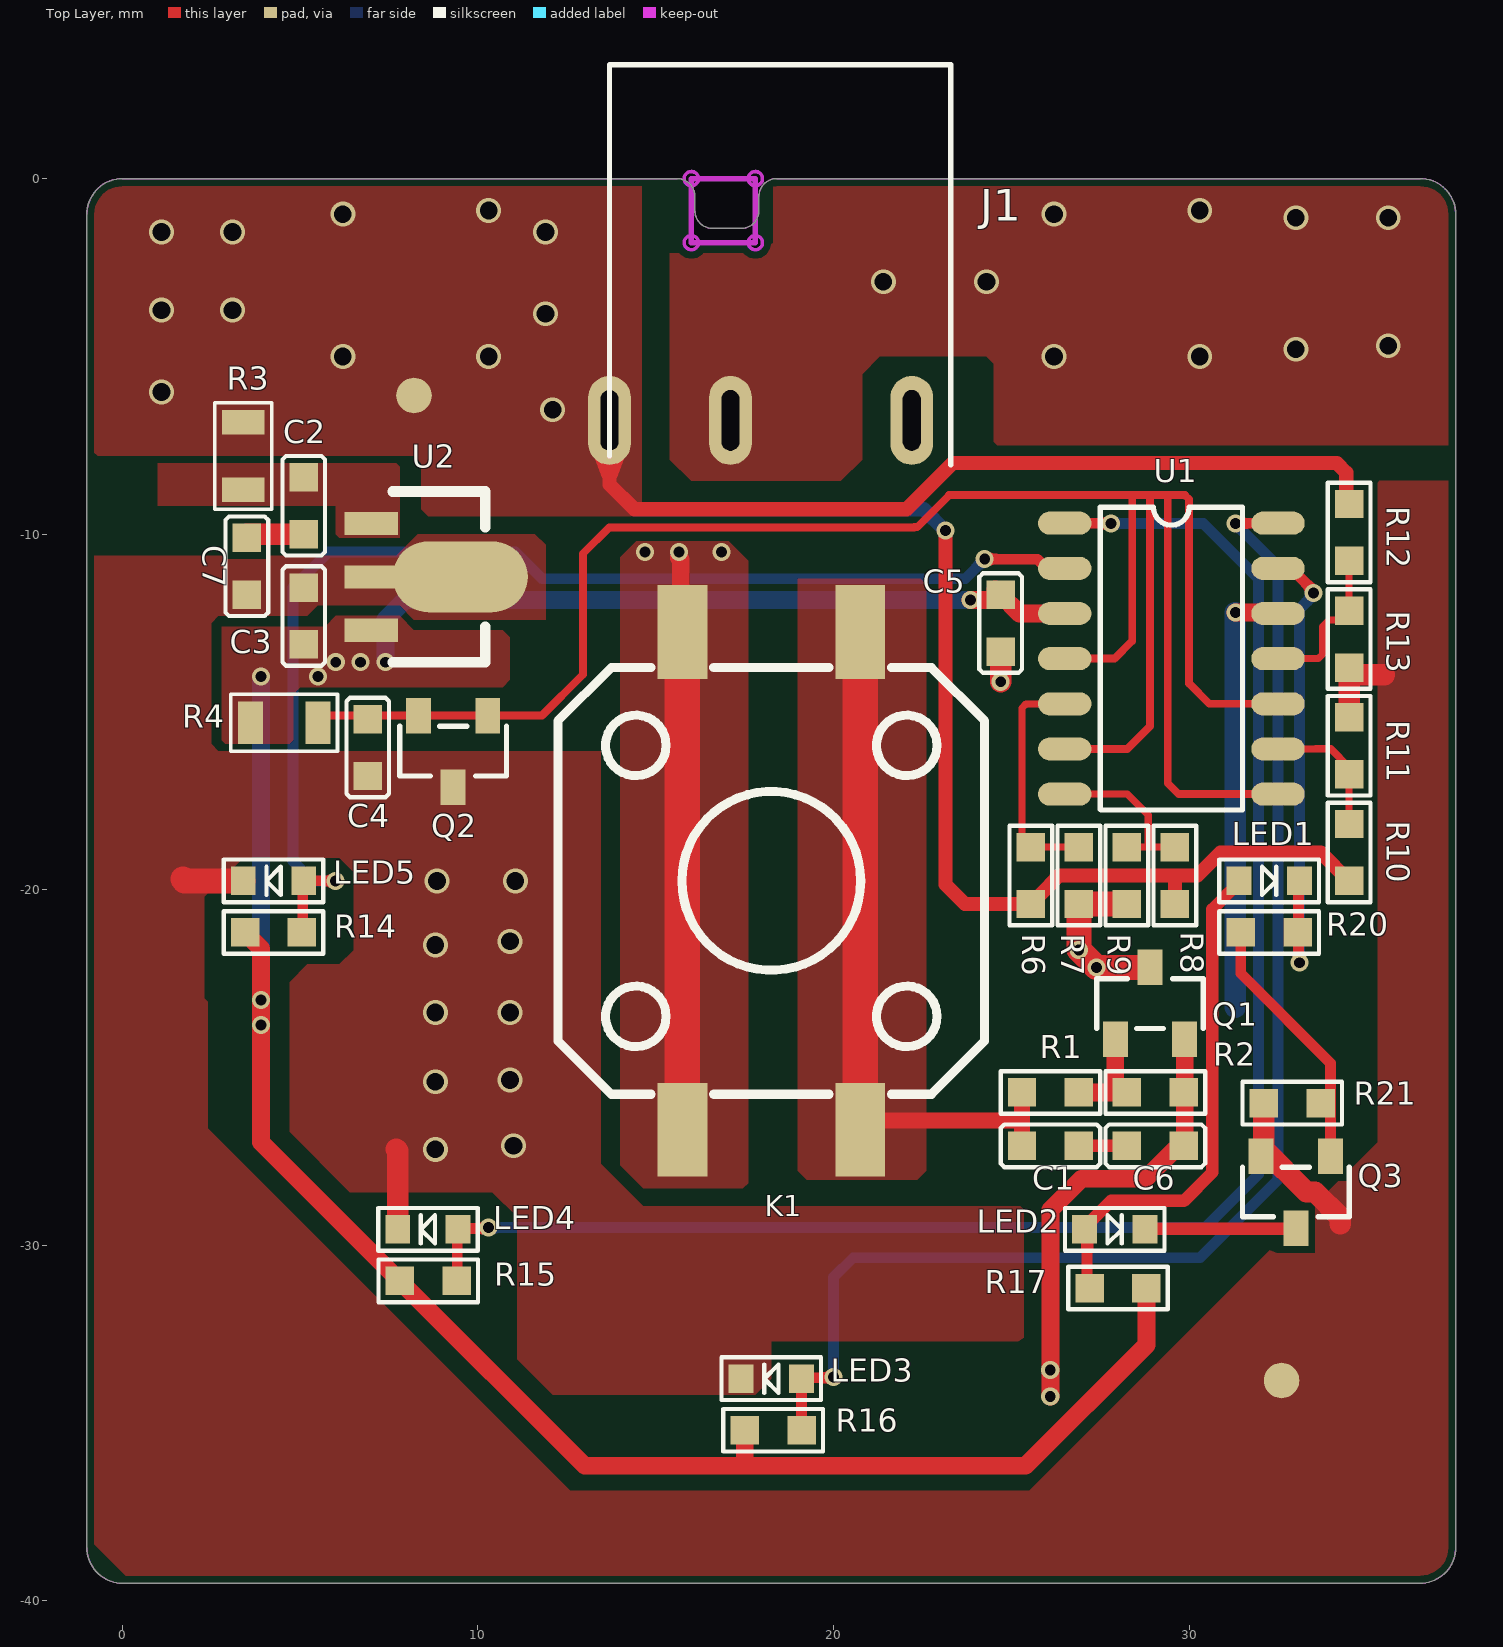
[diagram p0: Top Layer view]
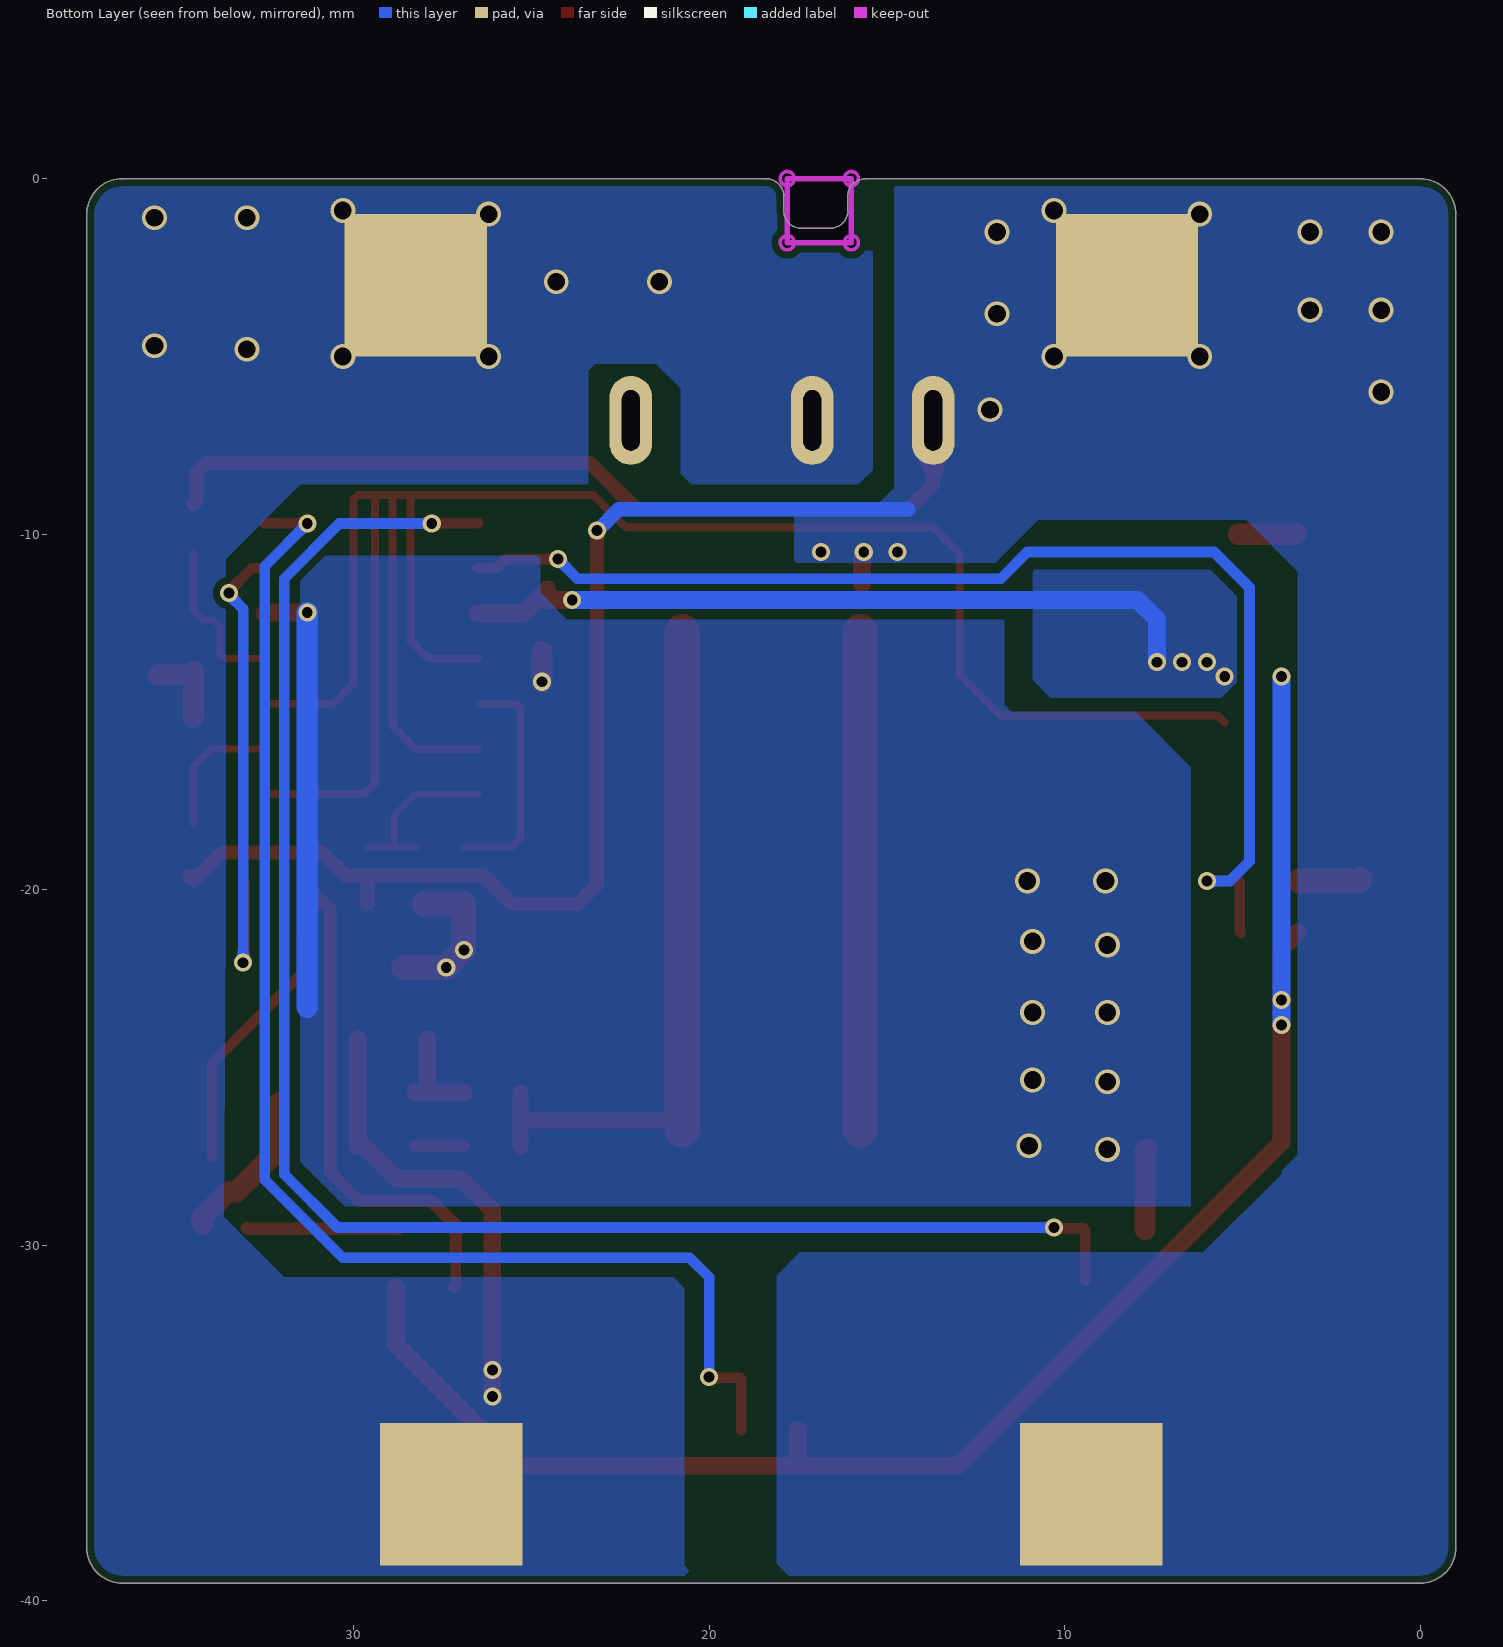
[diagram p1: Bottom Layer view, seen from below]
# Altium PCB MISC75799.PcbDoc
Units mm, origin at the board's own origin, x right, y up, seen from the top; angles counter-clockwise.
Board outline 38.5 x 39.5 mm, 2 copper layers (Top Layer, Bottom Layer); 37 components, 21 nets, 100 pads, 58 vias.

## Layer stack, top to bottom (the 12.6 mil dielectric is the usual default, probably not edited)
Top Solder: solder mask 0.0102, Solder Resist, Dk 3.5
Top Layer: signal copper 0.0356
Dielectric 1: dielectric 0.32, FR-4, Dk 4.8
Bottom Layer: signal copper 0.0356
Bottom Solder: solder mask 0.0102, Solder Resist, Dk 3.5

## Board outline
-1,-38.5 ccw(c0,-38.5) 0,-39.5 36.5,-39.5 ccw(c36.5,-38.5) 37.5,-38.5 37.5,-1 ccw(c36.5,-1) 36.5,0 18.4,0 ccw(c18.4,-0.5) 17.9,-0.5 17.9,-0.9 cw(c17.4,-0.9) 17.4,-1.4 16.6,-1.4 cw(c16.6,-0.9) 16.1,-0.9 16.1,-0.5 ccw(c15.6,-0.5) 15.6,0 0,0 ccw(c0,-1) -1,-1

## Design rules (kind name [scope] priority, off if disabled: settings)
Clearance [All] p1: gap=0.2 ignorepadtopadclearanceinfootprint=TRUE
MinimumSolderMaskSliver [All] p1: minsoldermaskwidth=0.01
PolygonConnect [All] p1: connectstyle=Direct reliefconductorwidth=0.254 reliefentries=4 polygonreliefangle="90 Angle" airgapwidth=0.254
RoutingVias [All] p1: holewidth=0.711 width=1.27 viastyle="Through Hole" minholewidth=0.711 minwidth=1.27 maxholewidth=0.711 maxwidth=1.27
SilkToSilkClearance [All] p1: silktosilkclearance=0
SilkToSolderMaskClearance [IsPad] p1: minsilkscreentomaskgap=0 clearancetoexposedcopper=TRUE
SolderMaskExpansion [All] p1: expansion=0.102 istentingtop=FALSE
SupplyNets "Schematic Supply Nets_4" [InNet('GND')] p1: voltage=0.000
SupplyNets "Schematic Supply Nets_3" [InNet('2.5V')] p2: voltage=0.000
SupplyNets "Schematic Supply Nets" [InNet('5V')] p3: voltage=0.000
Width [All] p1: maxlimit=1 minlimit=0.2 preferedwidth=0.3
27 further rules are at their usual default settings.

## Components (designator, comment, footprint, x,y, rotation, side; value= is the part's Value field where it differs from the comment)
C1 "1uF/50V" C0603A 26.1,-27.2 r0 top
C2 "1uF/50V" C0603A 5.1,-9.2 r90 top
C3 "1uF/50V" C0603A 5.1,-12.3 r270 top
C4 "1uF" C0603A 6.9,-16 r90 top
C5 "1uF" C0603A 24.7,-12.5 r90 top
C6 "1uF/50V" C0603A 29.05,-27.2 r0 top
C7 "1uF/50V" C0603A 3.5,-10.9 r90 top
J1 "DC-044/2.0芯卧插-耐高温260度" DC-044 18.5,-6.8 r0 top locked
K1 "SW-PB" SW-SMD_4P-L12.0-W12.0-P5.00-LS15.2 18.25,-19.75 r270 top locked
LED1 "Green" LED0603A 32.25,-19.75 r180 top locked
LED2 "Green" LED0603A 27.907,-29.55 r180 top locked
LED3 "Green" LED0603A 18.25,-33.75 r0 top locked
LED4 "Green" LED0603A 8.593,-29.55 r0 top locked
LED5 "Green" LED0603A 4.25,-19.75 r0 top locked
Q1 "2N7002K" SOT23-3 28.9,-23.2 r0 top
Q2 "TL431_23" SOT23-3 9.3,-16.1 r180 top
Q3 "2N7002" SOT23-3 33,-28.5 r180 top
R1 "3M" R0603A 26.1,-25.7 r0 top
R2 "1M" R0603A 29.05,-25.7 r0 top
R3 "100R" R0805A 3.4,-7.8 r90 top
R4 "2K" R0805A 4.55,-15.3 r180 top
R6 "145.2K" R0603A 25.55,-19.6 r270 top
R7 "10K 1%" R0603A 26.9,-19.6 r90 top
R8 "136.4K" R0603A 29.6,-19.6 r270 top
R9 "10K 1%" R0603A 28.25,-19.6 r90 top
R10 "128.4K" R0603A 34.5,-18.95 r270 top
R11 "10K 1%" R0603A 34.5,-15.95 r270 top
R12 "120K" R0603A 34.5,-9.95 r90 top
R13 "10K 1%" R0603A 34.5,-12.95 r90 top
R14 "1K" R0603A 4.25,-21.2 r0 top
R15 "1K" R0603A 8.6,-31 r0 top
R16 "1K" R0603A 18.3,-35.2 r0 top
R17 "1K" R0603A 28,-31.2 r180 top
R20 "100K" R0603A 32.25,-21.2 r0 top
R21 "1M" R0603A 32.9,-26 r0 top
U1 "LM339" SOP14L 29.5,-13.5 r0 top
U2 "DS8604" SOT-89-3 8.82,-11.2 r270 top

## Footprints (in the part's own frame and the unit in brackets; to place one, negate y for a bottom-side part, rotate by r counter-clockwise, add the part's x,y. Pads: shape width x height; smd on the part's side, far side on the other; paste and mask are expansions set on the pad)
C0603A [mm] "贴片电容"
  rect 0.8x0.8 smd mask+0.08: 1(-0.8,0) 2(0.8,0)
  silkscreen extent -1.4,-0.6 1.4,0.6
DC-044 [mm] "DC电源座直插-乐清市荆虹"
  oval 1.2x2.5 hole 0.5 slot 1.7 at 90 deg: 1(-4.8,0) 2(-1.4,0) 3(3.7,0)
  Keep-Out Layer board cut-out: -0.7,6.6 -0.777,6.615 -0.841,6.659 -0.885,6.723 -0.9,6.8 -0.9,6.8 -0.885,6.877 -0.841,6.941 -0.777,6.985 -0.7,7 -0.7,7 -0.623,6.985 -0.559,6.941 -0.515,6.877 -0.5,6.8 -0.5,6.8 -0.515,6.723 -0.559,6.659 -0.623,6.615 -0.7,6.6
  Keep-Out Layer board cut-out: -2.5,4.8 -2.577,4.815 -2.641,4.859 -2.685,4.923 -2.7,5 -2.7,5 -2.685,5.077 -2.641,5.141 -2.577,5.185 -2.5,5.2 -2.5,5.2 -2.423,5.185 -2.359,5.141 -2.315,5.077 -2.3,5 -2.3,5 -2.315,4.923 -2.359,4.859 -2.423,4.815 -2.5,4.8
  Keep-Out Layer board cut-out: -0.7,4.8 -0.777,4.815 -0.841,4.859 -0.885,4.923 -0.9,5 -0.9,5 -0.885,5.077 -0.841,5.141 -0.777,5.185 -0.7,5.2 -0.7,5.2 -0.623,5.185 -0.559,5.141 -0.515,5.077 -0.5,5 -0.5,5 -0.515,4.923 -0.559,4.859 -0.623,4.815 -0.7,4.8
  Keep-Out Layer board cut-out: -2.5,6.6 -2.577,6.615 -2.641,6.659 -2.685,6.723 -2.7,6.8 -2.7,6.8 -2.685,6.877 -2.641,6.941 -2.577,6.985 -2.5,7 -2.5,7 -2.423,6.985 -2.359,6.941 -2.315,6.877 -2.3,6.8 -2.3,6.8 -2.315,6.723 -2.359,6.659 -2.423,6.615 -2.5,6.6
  Keep-Out Layer board cut-out: -2.5,5 -2.5,6.8 -0.7,6.8 -0.7,5
  Keep-Out Layer circle w0.1: c-2.5,6.8 r0.2
  Keep-Out Layer circle w0.1: c-0.7,6.8 r0.2
  Keep-Out Layer circle w0.1: c-0.7,5 r0.2
  Keep-Out Layer circle w0.1: c-2.5,5 r0.2
  Keep-Out Layer lines w0.15: -2.5,5 -0.7,5 -0.7,6.8 -2.5,6.8 -2.5,5
  silkscreen extent -4.8,-1.25 4.8,10
LED0603A [mm] "贴片LED"
  rect 0.7x0.8 smd: 1(-0.85,0) 2(0.85,0)
  silkscreen extent -1.4,-0.6 1.4,0.6
R0603A [mm] "贴片电阻"
  rect 0.8x0.8 smd mask+0.08: 1(-0.8,0) 2(0.8,0)
  silkscreen extent -1.4,-0.6 1.4,0.6
R0805A [mm] "贴片电阻"
  rect 0.7x1.2 smd paste+0 mask+0.08: 1(-0.95,0) 2(0.95,0)
  silkscreen extent -1.5,-0.8 1.5,0.8
SOP14L [mm]
  oval 1.5x0.65 smd: 1(-3,3.81) 2(-3,2.54) 3(-3,1.27) 4(-3,0) 5(-3,-1.27) 6(-3,-2.54) 7(-3,-3.81) 8(3,-3.81) 9(3,-2.54) 10(3,-1.27) 11(3,0) 12(3,1.27) 13(3,2.54) 14(3,3.81)
  silkscreen extent -2,-4.26 2,4.26
SOT23-3 [mm] "贴片IC/MOS*"
  rect 0.7x1 smd: 1(-0.975,-1) 2(0.975,-1) 3(0,1.016)
  silkscreen extent -1.5,-0.7 1.5,0.7
SOT-89-3 [mm] "贴片线性稳压器"
  rect 0.65x1.5 smd mask+0.1: 1(-1.5,-1.82) 2(0,-1.82) 3(1.5,-1.82)
  oval 2x3.8 smd mask+0.1: 2(0,0.68)
  silkscreen extent -2.4,-1.22 2.4,1.38
SW-SMD_4P-L12.0-W12.0-P5.00-LS15.2 [mm]
  rect 2.64x1.4 smd: 1(-7,2.5) 1(7,2.5) 2(-7,-2.5) 2(7,-2.5)
  silkscreen extent -6,-6 6,6

## Part data
C1 C6: library part C0603, "0603 SMD capacitor"
C2 C3 C7: library part Cap, "Capacitor"
C4 C5: library part 0.1u
J1: "DC-044 power connector - Yueqing Jinghong"
K1: library part SW-PB_1, "6*6 tactile switch"
LED1 LED2 LED3 LED4 LED5: library part LED_Green, "SMD LED lamp"
Q1 Q3: library part NMOS
Q2: "IC SOT-23"
R1 R2 R6 R7 R8 R9 R10 R11 R12 R13 R21: library part R
R3 R4 R14 R15 R16 R17: library part RES
R20: library part R-S
U2: library part "LDO DS8604", "LDO"

## Free pads (board coordinates)
  rect 4x4 smd far side: 16(9.25,-37) 17(27.25,-37) 18(8.25,-3) 19(28.25,-3)
  round 1 smd: 20(8.2,-6.1) 21(32.6,-33.8)

## Via types
v1: diameter 0.7, hole 0.5, Top Layer to Bottom Layer, tented both sides, 32 vias
v2: diameter 0.508, hole 0.305, Top Layer to Bottom Layer, tented both sides, 26 vias

## Nets (pads, with @x,y where several pads share a name; then routed paths per layer and width w, separated by ;. In a path a pad name is that pad's centre, name@x,y a point inside that pad or via, vN(x,y) a via of type N, cw(c..) or ccw(c..) an arc to the next point about the centre after c; other vN are vias at no path point)
2.5V: C4.2 Q2.1 Q2.2 R4.1 U1.4 U1.6 U1.8 U1.10 | length 63.8
  Top Layer w0.22: R4.1 5.7,-15.1 Q2.2 Q2.1 11.8,-15.1 12.95,-13.95 12.95,-10.55 13.69,-9.81 22.261,-9.81 22.271,-9.8 22.35,-9.8 23.25,-8.9 28.4,-8.9 ; U1.6 28.26,-16.04 28.9,-15.4 28.9,-8.9 ; U1.4 27.9,-13.5 28.4,-13 28.4,-8.9 ; U1.8 29.71,-17.31 29.4,-17 29.4,-8.9 ; U1.10 30.57,-14.77 30,-14.2 30,-9.019 29.881,-8.9 29.4,-8.9 ; 28.4,-8.9 28.6,-8.9 28.9,-8.9 ; 28.9,-8.9 29.4,-8.9
5V: C3.2 C5.2 R4.2 R14.1 R15.1 R16.1 R17.1 U1.3 U2.3 | length 69.5
  Top Layer w0.5: R14.1 3.9,-21.65 v2(3.9,-23.1) v2(3.9,-23.8) 3.9,-27.1 R15.1 13,-36.2 17.5,-36.2 ; R16.1 17.5,-36.2 ; v2(23.85,-11.85) v2(23.85,-11.85) 24.55,-11.848 C5.2@24.55,-11.552 ; C5.2 25.23,-12.23 U1.3 ; R17.1 28.8,-32.8 25.4,-36.2 17.5,-36.2
  Bottom Layer w0.5: v2(3.9,-23.8) v2(3.9,-23.1) v2(3.9,-14) ; v2(7.4,-13.6) 7.4,-12.4 7.95,-11.85 v2(23.85,-11.85)
  other v2: 5.5,-14 6,-13.6 6.7,-13.6
GND: C3.1 C4.1 C5.1 C7.1 LED3.1 LED4.1 LED5.1 pad.21 Q1.3 Q2.3 Q3.2 R7.1 R9.1 R11.1 R13.1 R21.1 U1.12 U2.2 | length 28.2
  Top Layer w0.5: v2(31.3,-12.2) 31.302,-12.202 32.472,-12.202 U1.12
  Top Layer w0.6: 7.7,-27.3 7.743,-27.343 LED4.1 ; v2(24.7,-14.15) C5.1 ; R21.1 32.1,-27.3 33.3,-28.5 33.541,-28.5 34.25,-29.209 34.25,-29.4 ; R11.1 R13.1@34.5,-13.85 ; R13.1@34.5,-13.95 35.492,-13.95
  Top Layer w0.7: 1.7,-19.7 1.75,-19.75 LED5.1 ; R9.1@28,-20.4 R7.1 26.9,-21.687 27.397,-22.184 Q1.3@28.6,-22.184
  Bottom Layer w0.6: 31.3,-23.3 v2(31.3,-12.2)
  other v1: 8.8,-27.3 11,-27.2 8.8,-25.4 10.9,-25.35 8.8,-23.45 10.9,-23.45 8.8,-21.55 10.9,-21.45 8.85,-19.75 11.05,-19.75
  other v2: 27.392,-22.189 26.895,-21.692
NetC1_1: C1.1 K1.1 R1.1 | length 20.1
  Top Layer w0.45: K1.1@20.75,-26.75 21.013,-26.486 25.232,-26.486 ; C1.1 25.3,-26.486 R1.1
  Top Layer w1: K1.1@20.75,-26.75 K1.1@20.75,-12.75
NetC1_2: C1.2 C6.1 | length 1.3
  Top Layer w0.35: C1.2 C6.1
NetC2_1: C2.1 C7.2 | length 1.6
  Top Layer w0.6: C7.2@3.5,-10 C2.1
NetC2_2: C2.2 R3.1 U2.1
NetLED1_1: LED1.1 R20.2 U1.13 | length 14.2
  Top Layer w0.3: U1.13 32.866,-10.96 33.5,-11.594 v2(33.5,-11.65) ; LED1.1 33.075,-19.775 33.075,-21.125 33.1,-21.15 33.077,-21.173 33.077,-22.023 v2(33.104,-22.05)
  Bottom Layer w0.3: v2(33.104,-22.05) 33.104,-12.102 33.5,-11.706 v2(33.5,-11.65)
NetLED1_2: LED1.2 LED2.2 R17.2 | length 14.5
  Top Layer w0.3: 27.129,-30.15 27.129,-31.129 R17.2
  Top Layer w0.35: LED2.2 27.057,-29.5 27.807,-28.75 29.85,-28.75 30.65,-27.95 30.65,-20.55 31.4,-19.8 LED1.2 ; 27.129,-30.15 LED2.2@27.129,-29.55
NetLED2_1: LED2.1 Q3.3 | length 4.3
  Top Layer w0.35: LED2.1 28.774,-29.533 32.983,-29.533 Q3.3
NetLED3_2: LED3.2 R16.2 U1.14 | length 39
  Top Layer w0.3: R16.2 LED3.2 19.125,-33.725 19.975,-33.725 v2(20,-33.7) ; v2(31.3,-9.7) 31.305,-9.695 32.495,-9.695 U1.14
  Bottom Layer w0.3: v2(20,-33.7) 20,-30.9 20.55,-30.35 30.307,-30.35 32.5,-28.157 32.5,-10.9 v2(31.3,-9.7)
NetLED4_2: LED4.2 R15.2 U1.1 | length 47.5
  Top Layer w0.3: R15.2 9.421,-30.979 9.421,-29.571 9.468,-29.525 10.275,-29.525 v2(10.3,-29.5) ; U1.1 26.505,-9.695 27.795,-9.695 v2(27.8,-9.7)
  Bottom Layer w0.3: v2(10.3,-29.5) 30.45,-29.5 31.95,-28 31.95,-11.25 30.4,-9.7 v2(27.8,-9.7)
NetLED5_2: LED5.2 R14.2 U1.2 | length 34.3
  Top Layer w0.3: R14.2 5.075,-21.175 5.075,-19.775 LED5.2 v2@6,-19.75 ; v2(24.25,-10.7) 25.724,-10.7 25.984,-10.96 U1.2
  Bottom Layer w0.3: v2(5.995,-19.755) 5.355,-19.755 4.8,-19.2 4.8,-11.5 5.8,-10.5 11.05,-10.5 11.8,-11.25 23.7,-11.25 v2(24.25,-10.7)
NetQ1_1: Q1.1 R1.2 R2.1 | length 2.9
  Top Layer w0.5: R1.2 R2.1 ; Q1.1 27.925,-25.525 R2.1@28.1,-25.7
NetQ3_1: Q3.1 R20.1 R21.2 | length 7.3
  Top Layer w0.3: R20.1 31.45,-22.35 33.975,-24.875 33.975,-26 Q3.1
NetR6_1: R6.1 R7.2 U1.5 | length 6.6
  Top Layer w0.2: U1.5 25.417,-14.77 25.3,-14.887 25.3,-18.55 R6.1 R7.2
NetR8_1: R8.1 R9.2 U1.7 | length 4.8
  Top Layer w0.2: U1.7 28.26,-17.31 28.85,-17.9 28.85,-18.8 ; R9.2 28.85,-18.8 ; R8.1 28.85,-18.8
NetR10_1: R10.1 R11.2 U1.9 | length 3.8
  Top Layer w0.2: U1.9 33.554,-16.04 33.561,-16.033 33.983,-16.033 34.5,-16.55 R11.2 R10.1
NetR12_1: R12.1 R13.2 U1.11 | length 4.6
  Top Layer w0.2: U1.11 33.633,-13.5 33.75,-13.383 33.75,-12.6 33.938,-12.412 34.238,-12.412 R13.2 R12.1 R12.1@34.5,-10.55
P+: J1.1 K1.2 pad.16 pad.18 pad.20 R3.2 R6.2 R8.2 R10.2 R12.2 | length 71.6
  Top Layer w0.4: J1.1 13.7,-8.6 14.4,-9.3 22.05,-9.3 23.35,-8 34.15,-8 34.416,-8.266 34.416,-9.066 R12.2 ; v2(23.15,-9.896) 23.15,-19.85 23.7,-20.4 R6.2 26.1,-19.85 26.1,-19.834 26.334,-19.6 29.6,-19.6 ; R8.2 29.6,-19.6 ; R10.2@34.624,-19.626 R10.2 33.7,-18.95 30.884,-18.95 30.234,-19.6 29.6,-19.6
  Top Layer w0.5: v2@15.65,-10.66 15.7,-10.71 15.7,-11.4
  Top Layer w1: K1.2@15.75,-26.75 K1.2@15.75,-12.75
  Bottom Layer w0.4: 14.4,-9.3 22.538,-9.3 23.134,-9.896 v2(23.15,-9.896)
  other v1: 12.1,-6.5 1.1,-6 6.2,-5 10.3,-5 11.9,-3.8 1.1,-3.7 3.1,-3.7 1.1,-1.5 3.1,-1.5 11.9,-1.5 6.2,-1 10.3,-0.9
  other v2: 14.7,-10.5 15.65,-10.5 16.85,-10.5
P-: C6.2 J1.2 pad.17 pad.19 Q1.2 R2.2 | length 12.6
  Top Layer w0.5: v2@26.1,-34.247 26.1,-29 26.975,-28.125 28.775,-28.125 C6.2@29.7,-27.2 ; C6.2@29.875,-27.2 Q1.2
  other v1: 26.2,-5 30.3,-5 33,-4.8 35.6,-4.7 21.4,-2.9 24.3,-2.9 33,-1.1 35.6,-1.1 26.2,-1 30.3,-0.9
  other v2: 26.095,-34.252 26.095,-33.505
pads on no net: J1.3

## Polygon pours and split planes (outlines as drawn)
GND on Bottom Layer "NONET_L02_P-001" (solid, remove dead copper, pour order 8): 30.8,-10.6 31.5,-11.3 31.5,-27.65 30.25,-28.9 6.45,-28.9 6.45,-16.55 8,-15 11.5,-15 11.7,-14.8 11.7,-12.4 24,-12.4 24.75,-11.65 24.75,-10.5 24.85,-10.6
P- on Bottom Layer "NONET_L02_P-001" (solid, remove dead copper, pour order 1): 20.7,-31.2 21,-30.9 31.95,-30.9 33.65,-29.2 33.6,-21.2 33.6,-10.7 31.5,-8.6 23.4,-8.6 23.4,-5.4 23.2,-5.2 21.5,-5.2 20.8,-5.9 20.8,-8.3 20.5,-8.6 15.8,-8.6 15.4,-8.2 15.4,0 26.2,0 37.5,-0.1 37.5,-39.5 20.9,-39.5 20.55,-39.15 20.7,-39
5V on Bottom Layer "NONET_L02_P-001" (solid, remove dead copper, pour order 7): 5.1,-11.8 5.1,-14.1 5.6,-14.6 10.4,-14.6 10.9,-14.1 10.9,-11.1 11,-11 5.9,-11 5.7,-11.2
P+ on Bottom Layer "NONET_L02_P-001" (solid, remove dead copper, pour order 0): 14.8,-8.7 15.2,-9.1 17.35,-9.1 17.6,-9.35 17.6,-10.75 17.551,-10.8 11.95,-10.8 10.75,-9.6 4.9,-9.6 3.45,-11.05 3.45,-27.45 3.9,-27.9 3.9,-28 6.1,-30.2 17.45,-30.2 18.1,-30.85 18.1,-38.95 17.7,-39.35 17.65,-39.3 -0.5,-39.3 -0.7,-39.5 -1,-39.2 -1,0 14.8,0
GND on Top Layer "NONET_L02_P-001" (solid, remove dead copper, pour order 4): 2.3,-23.05 2.3,-20.2 3.4,-19.1 6.1,-19.1 6.5,-19.5 6.5,-21.7 6.1,-22.1 5.2,-22.1 4.7,-22.6 4.7,-26.8 6.4,-28.5 10.4,-28.5 11.1,-29.2 11.1,-33.2 12.1,-34.2 17.8,-34.2 18.25,-33.75 18.25,-32.7 25.35,-32.7 25.4,-32.65 25.35,-32.6 25.35,-29 25.25,-28.9 14.65,-28.9 13.45,-27.7 13.45,-16.1 2.7,-16.1 2.5,-15.9 2.5,-14.9 2.5,-12.5 2.7,-12.3 5.2,-12.3 5.5,-12 7.8,-12 8.2,-12.4 11.9,-12.4 11.9,-10.3 11.6,-10 8.3,-10 7.7,-10.6 -0.9,-10.6 -1,-10.7 -1,-38.2 0.3,-39.5 37.8,-39.5 37.8,-8.5 35.35,-8.5 35.3,-8.55 35.3,-27.1 25.5,-36.9 12.6,-36.9 2.4,-26.7 2.4,-23.15
P+ on Top Layer "NONET_L02_P-001" (solid, remove dead copper, pour order 10): 14,-10.65 14.45,-10.2 17.05,-10.2 17.6,-10.75 17.6,-28.25 17.45,-28.4 14.65,-28.4 14,-27.75
NetC1_1 on Top Layer "NONET_L02_P-001" (solid, remove dead copper, pour order 9): 19,-11.25 22.45,-11.25 22.6,-11.4 22.6,-27.9 22.35,-28.15 19.25,-28.15 19,-27.9
P- on Top Layer "NONET_L02_P-001" (solid, remove dead copper, pour order 6): 15.4,-2.1 15.4,-7.9 16,-8.5 20.2,-8.5 20.8,-7.9 20.8,-5.5 21.3,-5 24.3,-5 24.5,-5.2 24.5,-7.4 24.6,-7.5 37.6,-7.5 37.6,-7 37.5,-6.9 37.5,-0.1 37.3,0.1 18.5,0.1 18.3,-0.1 18.3,-1.8 18,-2.1 15.6,-2.1
NetC2_2 on Top Layer "NONET_L02_P-001" (solid, remove dead copper, pour order 3): 1,-9.2 1,-8 7.7,-8 7.8,-8.1 7.8,-10.1 6.1,-10.1 6,-10 6,-9.2
5V on Top Layer "NONET_L02_P-001" (solid, remove dead copper, pour order 5): 2.8,-15.8 2.9,-15.9 4.7,-15.9 4.8,-15.8 4.8,-14.5 5,-14.3 10.7,-14.3 10.9,-14.1 10.9,-12.9 10.7,-12.7 8.2,-12.7 7.8,-12.3 6,-12.3 5.7,-12.6 2.8,-12.6
P+ on Top Layer "NONET_L02_P-001" (solid, remove dead copper, pour order 2): 14.6,-9.2 14.3,-9.5 8.6,-9.5 8.4,-9.3 8.4,-8 8.2,-7.8 -0.7,-7.8 -1,-7.5 -1,0 14.6,0

## Keep-outs
Keep-Out Layer:
  lines w0.013: -1,-38.5 ccw(c0,-38.5) 0,-39.5 36.5,-39.5 ccw(c36.5,-38.5) 37.5,-38.5 37.5,-1 ccw(c36.5,-1) 36.5,0 35.5,0 18.4,0 ccw(c18.4,-0.5) 17.9,-0.5 17.9,-0.9 cw(c17.4,-0.9) 17.4,-1.4 16.6,-1.4 cw(c16.6,-0.9) 16.1,-0.9 16.1,-0.5 ccw(c15.6,-0.5) 15.6,0 1,0 0,0 ccw(c0,-1) -1,-1 -1,-38.5

## Silkscreen, mask and mechanical layers (free items; w line width, h text height)
Mechanical 1:
  drawing of 189 lines, arcs and shapes, not listed
  text "LED}5" at 5.585,-20.07 h1
  text "LED}1" at 27.871,-20.152 h1
  text "LED}2" at 29.213,-30.069 h1
  text "LED}4" at 10.227,-30.153 h1
  text "LED}3" at 19.627,-34.231 h1
Mechanical 3:
  drawing of 176 lines, arcs and shapes, not listed